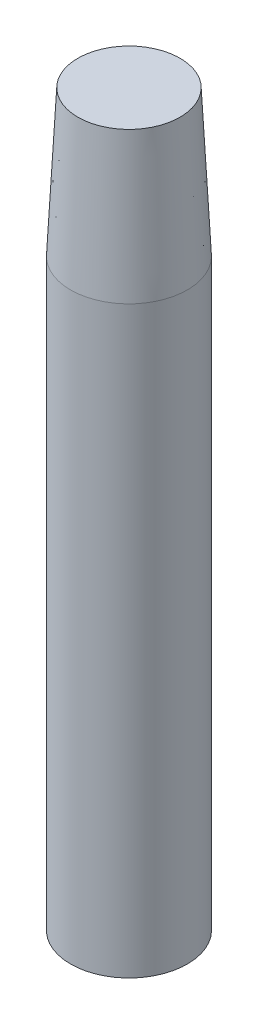
from build123d import *

# Parameters (mm, degrees)
SKETCH1_R             = 4
BOSS_EXTRUDE1_DEPTH   = 50
CHAMFER1_SIZE         = 10
CHAMFER1_SIZE2        = 0.5
M4_TAPPED_HOLE1_D     = 3.3
M4_TAPPED_HOLE1_DEPTH = 10.1
M4_TAPPED_HOLE1_TIP   = 0.991420021


with BuildPart() as part:
    # Sketch1 → Boss-Extrude1 (new body)
    with BuildSketch(Plane(origin=(0, 0, 0), x_dir=(1, 0, 0), z_dir=(0, 1, 0))):
        with Locations(Location((0, 0, 0), (0, 0, 270))):
            Circle(SKETCH1_R)
    extrude(amount=BOSS_EXTRUDE1_DEPTH)

    # Chamfer1
    chamfer1_edges = [part.edges().sort_by_distance(p)[0] for p in [
        (0, 50, -4),
    ]]
    chamfer1_side = [part.faces().sort_by_distance(p)[0] for p in [
        (0, 25, -4),
    ]]
    chamfer(chamfer1_edges, length=CHAMFER1_SIZE, length2=CHAMFER1_SIZE2, reference=chamfer1_side[0])

    # M4 Tapped Hole1
    with Locations(Plane(origin=(0, 0, 0), x_dir=(-1, 0, 0), z_dir=(0, -1, 0))):
        with Locations((0, 0)):
            Hole(M4_TAPPED_HOLE1_D / 2, depth=M4_TAPPED_HOLE1_DEPTH)
            with Locations((0, 0, -(M4_TAPPED_HOLE1_DEPTH + M4_TAPPED_HOLE1_TIP / 2))):  # 118° drill point
                Cone(0, M4_TAPPED_HOLE1_D / 2, M4_TAPPED_HOLE1_TIP, mode=Mode.SUBTRACT)


solid = part.part
